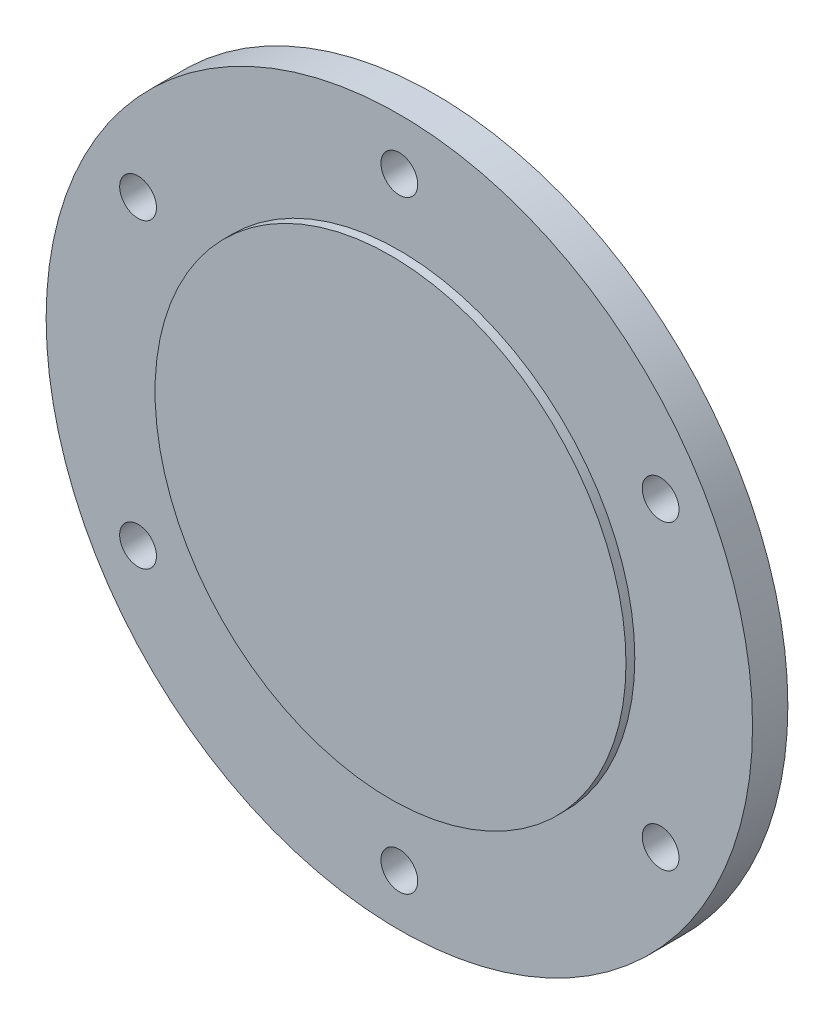
from build123d import *

# Parameters (mm, degrees)
SKETCH1_W                         = 120
SKETCH1_H                         = 12
SKETCH2_R                         = 85
BOSS_EXTRUDE1_DEPTH               = 2.5
SKETCH3_R                         = 80
BOSS_EXTRUDE2_DEPTH               = 3
F_12_5_12_5_DIAMETER_HOLE1_D      = 12.5
F_12_5_12_5_DIAMETER_HOLE1_DEPTH  = 14.5
M90_COUNTERBORE_HOLE1_D           = 100
M90_COUNTERBORE_HOLE1_CBORE_D     = 130
M90_COUNTERBORE_HOLE1_CBORE_DEPTH = 1
SKETCH8_R                         = 50.101943112
BOSS_EXTRUDE3_DEPTH               = 7


with BuildPart() as part:
    # Sketch1 → Revolve1 (revolve)
    with BuildSketch(Plane(origin=(0, 234.743963655, 0), x_dir=(1, 0, 0), z_dir=(0, 1, 0))):
        with Locations((581.230642584, 144.692981355)):
            Rectangle(SKETCH1_W, SKETCH1_H)
    revolve(axis=Axis((521.230642584, 234.743963655, -150.692981355), (0, 0, 1)))

    # Sketch2 → Boss-Extrude1 (add)
    with BuildSketch(Plane(origin=(0, 0, -150.692981355), x_dir=(-1, 0, 0), z_dir=(0, 0, -1))):
        with Locations((-521.230642584, 234.743963655)):
            Circle(SKETCH2_R)
    extrude(amount=BOSS_EXTRUDE1_DEPTH)

    # Sketch3 → Boss-Extrude2 (add)
    with BuildSketch(Plane.XY.offset(-138.692981355)):
        with Locations((521.230642584, 234.743963655)):
            Circle(SKETCH3_R)
    extrude(amount=BOSS_EXTRUDE2_DEPTH)

    # Ø12.5 (12.5) Diameter Hole1
    with Locations(Plane.XY.offset(-138.692981355)):
        with Locations((521.230642584, 337.243963655), (609.998246472, 285.993963655), (432.463038696, 285.993963655), (432.463038696, 183.493963655), (521.230642584, 132.243963655), (609.998246472, 183.493963655)):
            Hole(F_12_5_12_5_DIAMETER_HOLE1_D / 2, depth=F_12_5_12_5_DIAMETER_HOLE1_DEPTH)

    # M90 counterbore hole1 (through all)
    with Locations(Plane(origin=(0, 0, -153.192981355), x_dir=(-1, 0, 0), z_dir=(0, 0, -1))):
        with Locations((-521.230642584, 234.743963655)):
            CounterBoreHole(M90_COUNTERBORE_HOLE1_D / 2, M90_COUNTERBORE_HOLE1_CBORE_D / 2, M90_COUNTERBORE_HOLE1_CBORE_DEPTH)

    # Sketch8 → Boss-Extrude3 (add)
    with BuildSketch(Plane.XY.offset(-135.692981355)):
        with Locations((521.230642584, 234.743963655)):
            Circle(SKETCH8_R)
    extrude(amount=-BOSS_EXTRUDE3_DEPTH)


solid = part.part
